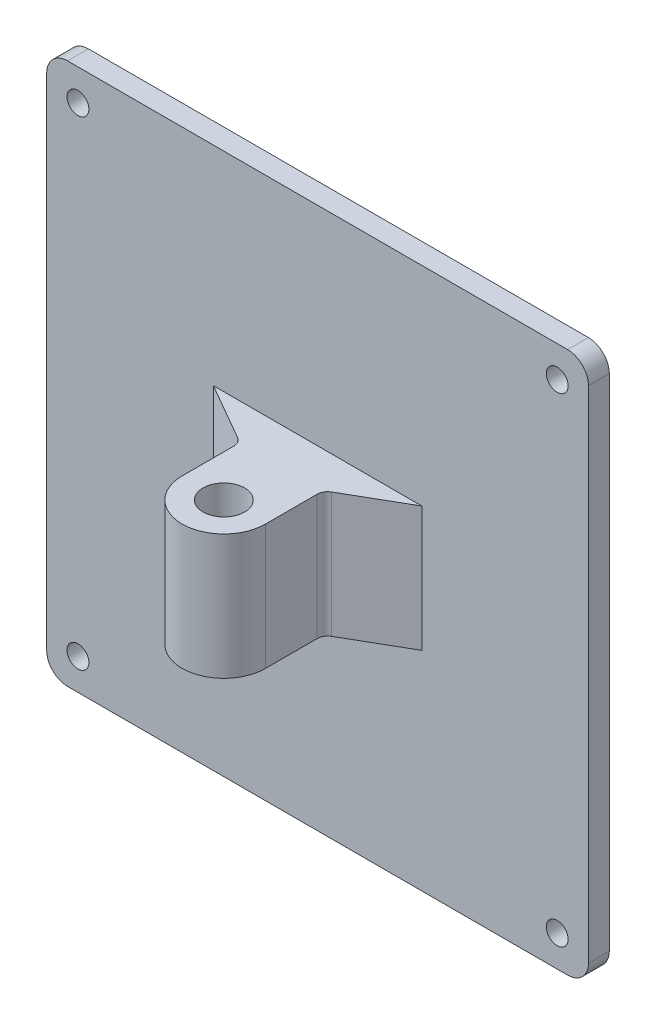
from build123d import *

# Parameters (mm, degrees)
SKETCH_1_R          = 5.25
EXTRUDE_1_DEPTH     = 10
EXTRUDE_2_DEPTH     = 30
SKETCH_3_R          = 10
CUT_EXTRUDE_1_DEPTH = 134
FILLET_1_R          = 5


with BuildPart() as part:
    # 草图1 → 凸台-拉伸1 (new body)
    with BuildSketch(Plane.XY):
        with BuildLine():
            Line((-120, -130), (120, -130))
            ThreePointArc((120, -130), (127.071067812, -127.071067812), (130, -120))
            Line((130, -120), (130, 120))
            ThreePointArc((130, 120), (127.071067812, 127.071067812), (120, 130))
            Line((120, 130), (-120, 130))
            ThreePointArc((-120, 130), (-127.071067812, 127.071067812), (-130, 120))
            Line((-130, 120), (-130, -120))
            ThreePointArc((-130, -120), (-127.071067812, -127.071067812), (-120, -130))
        make_face()
        with Locations((-115, 115)):
            Circle(SKETCH_1_R, mode=Mode.SUBTRACT)
        with Locations((115, 115)):
            Circle(SKETCH_1_R, mode=Mode.SUBTRACT)
        with Locations((115, -115)):
            Circle(SKETCH_1_R, mode=Mode.SUBTRACT)
        with Locations((-115, -115)):
            Circle(SKETCH_1_R, mode=Mode.SUBTRACT)
    extrude(amount=EXTRUDE_1_DEPTH)

    # 草图2 → 凸台-拉伸2 (add, symmetric)
    with BuildSketch(Plane(origin=(0, 0, 0), x_dir=(1, 0, 0), z_dir=(0, 1, 0))):
        with BuildLine():
            Line((-50, -10), (50, -10))
            Line((50, -10), (20, -27.278852826))
            Line((20, -27.278852826), (20, -55))
            ThreePointArc((20, -55), (0, -75), (-20, -55))
            Line((-20, -55), (-20, -27.278852826))
            Line((-20, -27.278852826), (-50, -10))
        make_face()
    extrude(amount=EXTRUDE_2_DEPTH, both=True)

    # 草图3 → 切除-拉伸1 (cut)
    with BuildSketch(Plane.XZ.offset(30)):
        with Locations(Location((0, 55, 0), (0, 0, 270))):
            Circle(SKETCH_3_R)
    extrude(amount=-CUT_EXTRUDE_1_DEPTH, mode=Mode.SUBTRACT)

    # 圆角1
    fillet_1_edges = [part.edges().sort_by_distance(p)[0] for p in [
        (-20, 0, 27.278852826),
        (20, 0, 27.278852826),
    ]]
    fillet(fillet_1_edges, radius=FILLET_1_R)


solid = part.part
